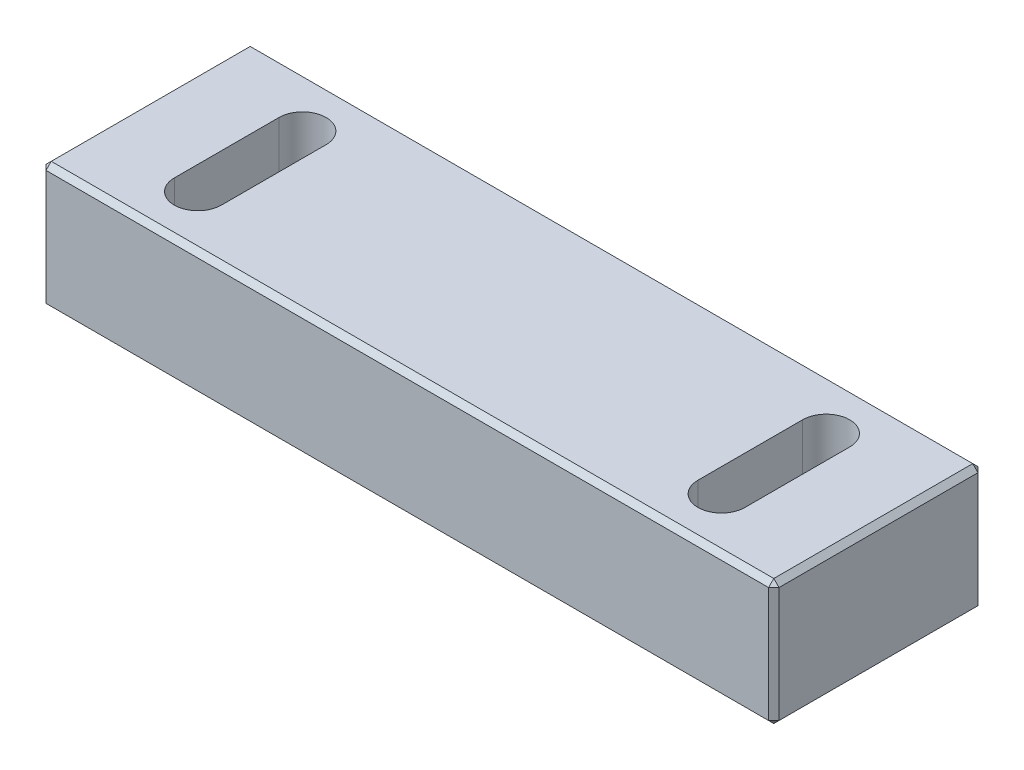
SolidWorks part; units mm, degrees
material "45#"
ref_plane "Front Plane" through (0, 0, 0) normal (0, 0, 1) x (1, 0, 0)
ref_plane "Top Plane" through (0, 0, 0) normal (0, 1, 0) x (1, 0, 0)
ref_plane "Right Plane" through (0, 0, 0) normal (1, 0, 0) x (0, 0, -1)
sketch "Sketch1" plane through (0, 0, 0) normal (0, 1, 0) x (1, 0, 0)
  line L0 (-35, 10) -> (35, -10) construction
  line L1 (-35, 10) -> (35, 10)
  line L2 (-35, 10) -> (-35, -10)
  line L3 (-35, -10) -> (35, -10)
  line L4 (35, 10) -> (35, -10)
  dimension "D1" = 70
  dimension "D2" = 20
extrude "Extrude1" add sketch "Sketch1" along normal blind 12
sketch "Sketch2" plane through (0, 12, 0) normal (0, 1, 0) x (1, 0, 0)
  line L0 (0, 10) -> (0, -10) construction
  line L1 (22.75, 5) -> (22.75, -5)
  line L2 (-27.25, 5) -> (-27.25, -5)
  line L3 (27.25, 5) -> (27.25, -5)
  line L4 (-22.75, 5) -> (-22.75, -5)
  line L5 (35, 10) -> (-35, 10) construction
  line L6 (-35, -10) -> (35, -10) construction
  line L7 (0, 0) -> (-22.75, 0) construction
  arc A0 (-27.25, 5) -> (-22.75, 5) centre (-25, 5) cw
  arc A1 (-22.75, -5) -> (-27.25, -5) centre (-25, -5) cw
  arc A2 (22.75, -5) -> (27.25, -5) centre (25, -5) ccw
  arc A3 (27.25, 5) -> (22.75, 5) centre (25, 5) ccw
  dimension "D1" = 50
  dimension "D2" = 4.5
  dimension "D3" = 10
extrude "Cut-Extrude1" cut sketch "Sketch2" against normal through all
chamfer "Chamfer1" distance 0.5 angle 45 12 edges at (0, 12, 10) (35, 6, 10) (35, 12, 0) (35, 6, -10) (0, 12, -10) (-35, 6, -10) (-35, 12, 0) (-35, 6, 10) (0, 0, 10) (35, 0, 0) (0, 0, -10) (-35, 0, 0)
